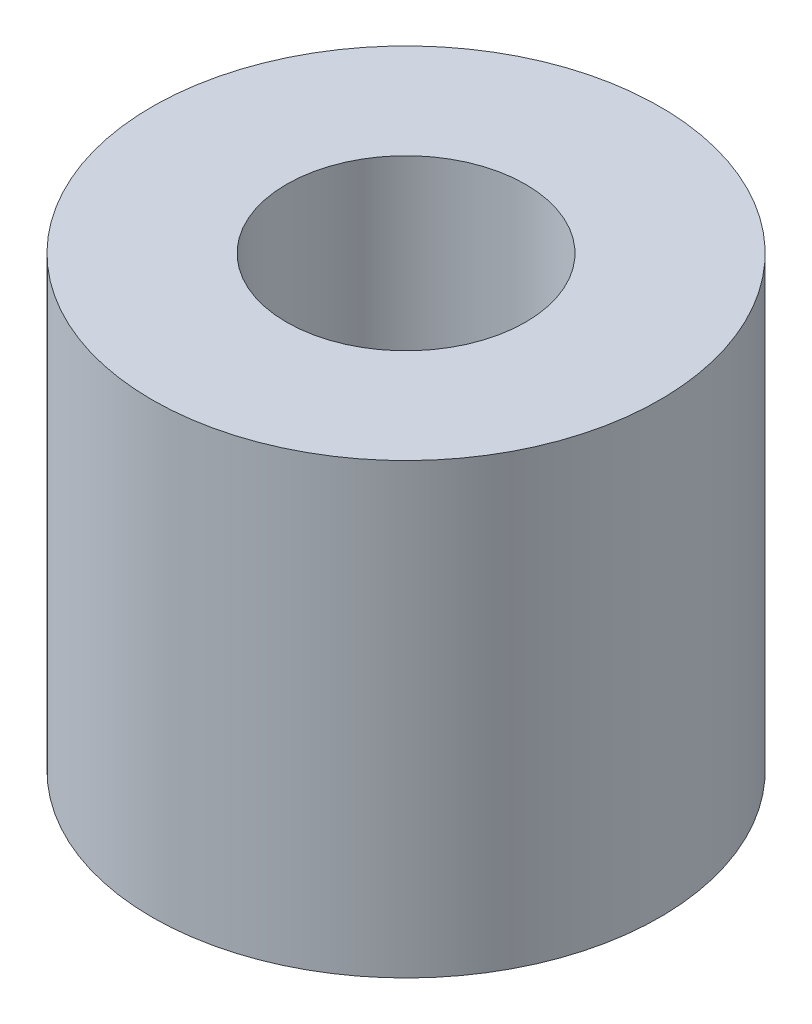
from build123d import *

# Parameters (mm, degrees)
SKETCH_1_R      = 3.4
SKETCH_1_R_2    = 1.6
EXTRUDE_1_DEPTH = 6


with BuildPart() as part:
    # 草图1 → 凸台-拉伸1 (new body)
    with BuildSketch(Plane(origin=(0, 0, 0), x_dir=(1, 0, 0), z_dir=(0, 1, 0))):
        with Locations(Location((0, 0, 0), (0, 0, 270))):
            Circle(SKETCH_1_R)
        with Locations(Location((0, 0, 0), (0, 0, 270))):
            Circle(SKETCH_1_R_2, mode=Mode.SUBTRACT)
    extrude(amount=EXTRUDE_1_DEPTH)


solid = part.part
